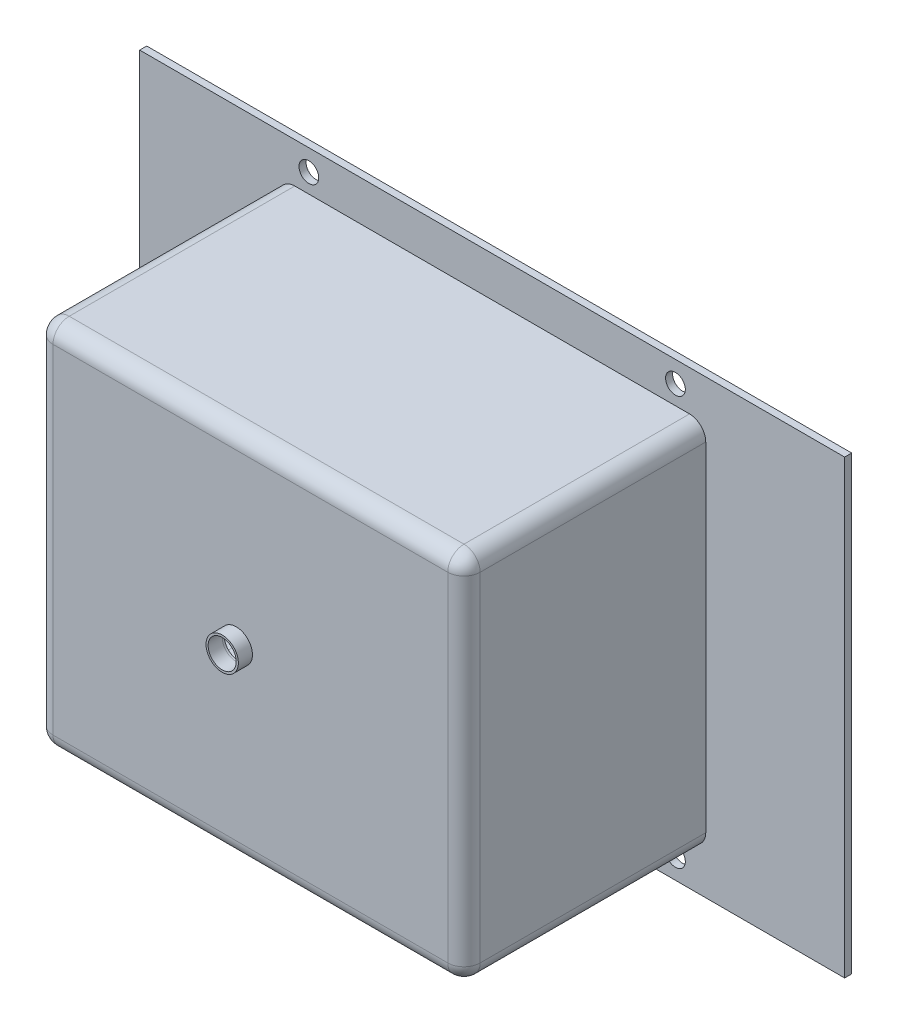
SolidWorks part; units mm, degrees
ref_plane "Front Plane" through (0, 0, 0) normal (0, 0, 1) x (1, 0, 0)
ref_plane "Top Plane" through (0, 0, 0) normal (0, 1, 0) x (1, 0, 0)
ref_plane "Right Plane" through (0, 0, 0) normal (1, 0, 0) x (0, 0, -1)
other "Configuration Table"
sketch "Sketch1" plane through (0, 0, 0) normal (0, 0, 1) x (1, 0, 0)
  line L1 (0, 0) -> (300, 0)
  line L2 (0, 0) -> (0, 260)
  line L3 (0, 260) -> (300, 260)
  line L4 (300, 0) -> (300, 260)
  line L9 (-100, 290) -> (400, 290)
  line L10 (-100, 290) -> (-100, -30)
  line L11 (-100, -30) -> (400, -30)
  line L12 (400, 290) -> (400, -30)
  point P9 (300, 130)
  dimension "D1" = 260
  dimension "D2" = 300
  dimension "D3" = 30
  dimension "D4" = 30
  dimension "D5" = 100
  dimension "D6" = 100
extrude "Boss-Extrude1" add sketch "Sketch1" along normal blind 5
sketch "Sketch2" plane through (0, 0, 5) normal (0, 0, 1) x (1, 0, 0)
  line L1 (0, 260) -> (300, 260)
  line L2 (0, 260) -> (0, 0)
  line L3 (0, 0) -> (300, 0)
  line L4 (300, 260) -> (300, 0)
  line L5 (-1.5, 261.5) -> (301.5, 261.5)
  line L6 (-1.5, 261.5) -> (-1.5, -1.5)
  line L7 (-1.5, -1.5) -> (301.5, -1.5)
  line L8 (301.5, 261.5) -> (301.5, -1.5)
  dimension "D1" = 1.5
  dimension "D2" = 1.5
  dimension "D3" = 1.5
  dimension "D4" = 1.5
extrude "Boss-Extrude2" add sketch "Sketch2" along normal blind 170
sketch "Sketch3" plane through (0, 0, 175) normal (0, 0, 1) x (1, 0, 0)
  line L1 (301.5, 261.5) -> (-1.5, 261.5)
  line L2 (301.5, 261.5) -> (301.5, -1.5)
  line L3 (301.5, -1.5) -> (-1.5, -1.5)
  line L4 (-1.5, 261.5) -> (-1.5, -1.5)
  circle A0 centre (140, 130) radius 10
  dimension "D1" = 20
extrude "Boss-Extrude3" add sketch "Sketch3" along normal blind 1.5
fillet "Fillet2" radius 10 8 edges at (300, 260, 87.5) (0, 260, 87.5) (150, 260, 175) (300, 130, 175) (300, 0, 87.5) (0, 0, 87.5) (150, 0, 175) (0, 130, 175)
fillet "Fillet3" radius 11.5 8 edges at (301.5, 130, 176.5) (301.5, 261.5, 90.75) (301.5, -1.5, 90.75) (-1.5, -1.5, 90.75) (150, -1.5, 176.5) (-1.5, 130, 176.5) (150, 261.5, 176.5) (-1.5, 261.5, 90.75)
sketch "Sketch4" plane through (0, 0, 176.5) normal (0, 0, 1) x (1, 0, 0)
  circle A0 centre (140, 130) radius 9.9677
  circle A1 centre (140, 130) radius 11.4677
  dimension "D1" = 1.5
extrude "Boss-Extrude4" add sketch "Sketch4" along normal blind 10
sketch "Sketch5" plane through (0, 0, 0) normal (0, 0, -1) x (-1, 0, 0)
  line L0 (-290, 260) -> (-10, 260) construction
  line L1 (100, -30) -> (-400, -30) construction
  line L2 (100, 290) -> (100, -30) construction
  line L3 (-400, -30) -> (-400, 290) construction
  circle A0 centre (-20, -15) radius 7
  circle A1 centre (-280, -15) radius 7
  circle A2 centre (-20, 275) radius 7
  circle A3 centre (-280, 275) radius 7
  dimension "D1" = 14
  dimension "D2" = 14
  dimension "D3" = 14
  dimension "D4" = 14
  dimension "D5" = 15
  dimension "D6" = 15
  dimension "D7" = 15
  dimension "D8" = 15
  dimension "D9" = 120
  dimension "D10" = 120
  dimension "D11" = 120
  dimension "D12" = 120
extrude "Cut-Extrude1" cut sketch "Sketch5" against normal through all
sketch "Sketch6" plane through (0, 0, 0) normal (0, 0, -1) x (-1, 0, 0)
  circle A0 centre (56.636, 245.0886) radius 10.6661
  circle A1 centre (56.636, 210.0886) radius 10.6661
  circle A2 centre (56.636, 175.0886) radius 10.6661
  dimension "D1" = 3
extrude "Boss-Extrude5" add sketch "Sketch6" along normal blind 2
